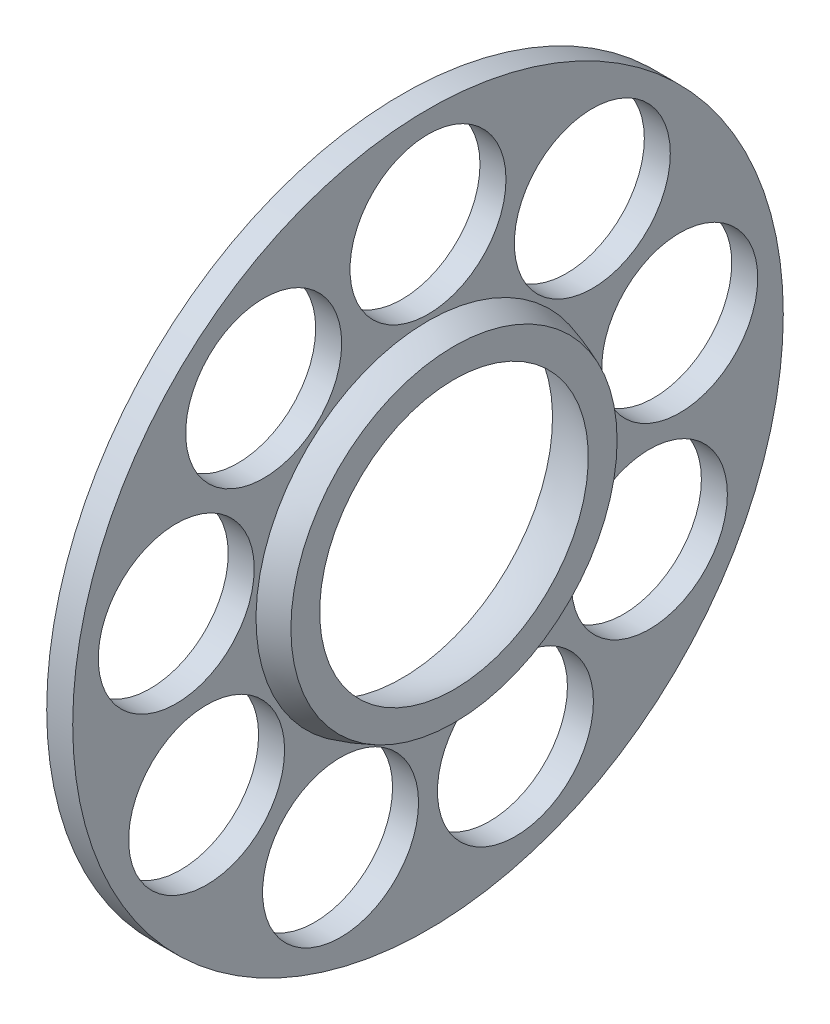
from build123d import *

# Parameters (mm, degrees)
SKETCH4_R          = 9
CUT_EXTRUDE1_DEPTH = 10


with BuildPart() as part:
    # Sketch2 → Revolve1 (revolve)
    with BuildSketch(Plane.XY):
        with BuildLine():
            Line((6, 0), (6, 18.821530225))
            ThreePointArc((6, 18.821530225), (4.519902914, 19.393505195), (3, 19.849287907))
            Line((3, 19.849287907), (3, 41))
            Line((3, 41), (0, 41))
            Line((0, 41), (0, 0))
            Line((0, 0), (6, 0))
        make_face()
    revolve(axis=Axis((0, 0, 0), (1, 0, 0)))

    # Sketch3 → Cut-Revolve1 (revolve, cut)
    with BuildSketch(Plane.XY, mode=Mode.PRIVATE) as cut_revolve1_sk:
        with BuildLine():
            Line((6, 15.5), (6, 0))
            Line((6, 0), (0, 0))
            Line((0, 0), (0, 17.370620624))
            ThreePointArc((0, 17.370620624), (3.084663444, 16.706867601), (6, 15.5))
        make_face()
    revolve(cut_revolve1_sk.sketch.rotate(Axis((6, 0, 0), (-1, 0, 0)), 270), axis=Axis((6, 0, 0), (-1, 0, 0)), mode=Mode.SUBTRACT)

    # Sketch4 → Cut-Extrude1 (cut)
    with BuildSketch(Plane(origin=(3, 0, 0), x_dir=(0, 0, -1), z_dir=(1, 0, 0))):
        with Locations((0, 29.5)):
            Circle(SKETCH4_R)
        with Locations((18.962234486, 22.598311072)):
            Circle(SKETCH4_R)
        with Locations((29.051828714, 5.122621241)):
            Circle(SKETCH4_R)
        with Locations((25.547749412, -14.75)):
            Circle(SKETCH4_R)
        with Locations((10.089594228, -27.720932313)):
            Circle(SKETCH4_R)
        with Locations((-10.089594228, -27.720932313)):
            Circle(SKETCH4_R)
        with Locations((-25.547749412, -14.75)):
            Circle(SKETCH4_R)
        with Locations((-29.051828714, 5.122621241)):
            Circle(SKETCH4_R)
        with Locations((-18.962234486, 22.598311072)):
            Circle(SKETCH4_R)
    extrude(amount=-CUT_EXTRUDE1_DEPTH, mode=Mode.SUBTRACT)


solid = part.part
